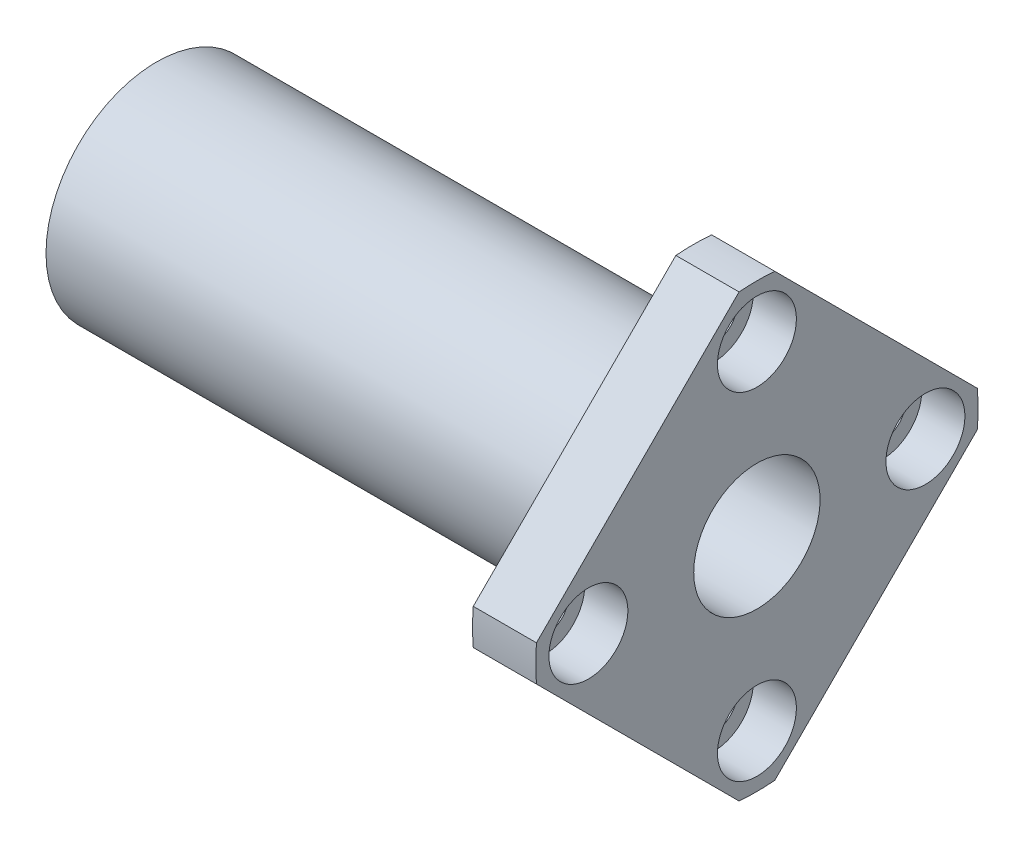
SolidWorks part; units mm, degrees
ref_plane "Front Plane" through (0, 0, 0) normal (0, 0, 1) x (1, 0, 0)
ref_plane "Top Plane" through (0, 0, 0) normal (0, 1, 0) x (1, 0, 0)
ref_plane "Right Plane" through (0, 0, 0) normal (1, 0, 0) x (0, 0, -1)
sketch "Sketch1" plane through (0, 0, 0) normal (1, 0, 0) x (0, 0, -1)
  circle A0 centre (0, 0) radius 6
  circle A1 centre (0, 0) radius 10.5
extrude "Boss-Extrude1" add sketch "Sketch1" along normal mid plane 57
sketch "Sketch2" plane through (28.5, 0, 0) normal (1, 0, 0) x (0, 0, -1)
  circle A0 centre (0, 0) radius 6
  circle A1 centre (0, 0) radius 21
extrude "Boss-Extrude2" add sketch "Sketch2" against normal blind 6
hole_wizard "Ø7.5 (7.5) Diameter Hole1" positions "Sketch4" profile "Sketch3" hole size "Ø7.5" standard "GB"
sketch "Sketch4" plane through (28.5, 0, 0) normal (1, 0, 0) x (0, 0, -1)
  point P0 (0, 16)
sketch "Sketch3" plane through (28.5, 16, 0) normal (0, 1, 0) x (0, 0, -1)
  line L0 (0, 0) -> (0, 4.1)
  line L1 (0, 4.1) -> (3.75, 4.1)
  line L2 (3.75, 4.1) -> (3.75, 0)
  line L5 (3.75, 0) -> (0, 0)
  line L10 (0, 4.1) -> (-3.75, 4.1) construction
  line L11 (0, -6.35) -> (0, 107.95) construction
  dimension "孔直径" = 7.5
  dimension "孔深度" = 4.1
  dimension "导头角度" = 180
hole_wizard "Ø4.5 (4.5) Diameter Hole1" positions "Sketch6" profile "Sketch5" hole size "Ø4.5" standard "GB" end condition up to next
sketch "Sketch6" plane through (24.4, 0, 0) normal (1, 0, 0) x (0, 0, -1)
  point P0 (0, 16)
sketch "Sketch5" plane through (24.4, 16, 0) normal (0, 1, 0) x (0, 0, -1)
  line L0 (0, 0) -> (0, 1.901)
  line L1 (0, 1.901) -> (2.25, 1.901)
  line L2 (2.25, 1.901) -> (2.25, 0)
  line L5 (2.25, 0) -> (0, 0)
  line L11 (0, -6.35) -> (0, 107.95) construction
  dimension "通孔孔直径" = 4.5
  dimension "通孔孔深度" = 1.901
pattern_circular "CirPattern1" count 4 over 360 about axis through (0, 0, 0) along (1, 0, 0) of "Ø4.5 (4.5) Diameter Hole1", "Ø7.5 (7.5) Diameter Hole1"
sketch "Sketch7" plane through (28.5, 0, 0) normal (1, 0, 0) x (0, 0, -1)
  line L0 (0, 22.6274) -> (-22.6274, 0)
  line L1 (-22.6274, 0) -> (0, -22.6274)
  line L2 (0, -22.6274) -> (22.6274, 0)
  line L3 (22.6274, 0) -> (0, 22.6274)
  dimension "D1" = 16
  dimension "D2" = 16
  dimension "D3" = 16
  dimension "D4" = 16
extrude "Cut-Extrude1" cut sketch "Sketch7" against normal up to next flip side to cut
